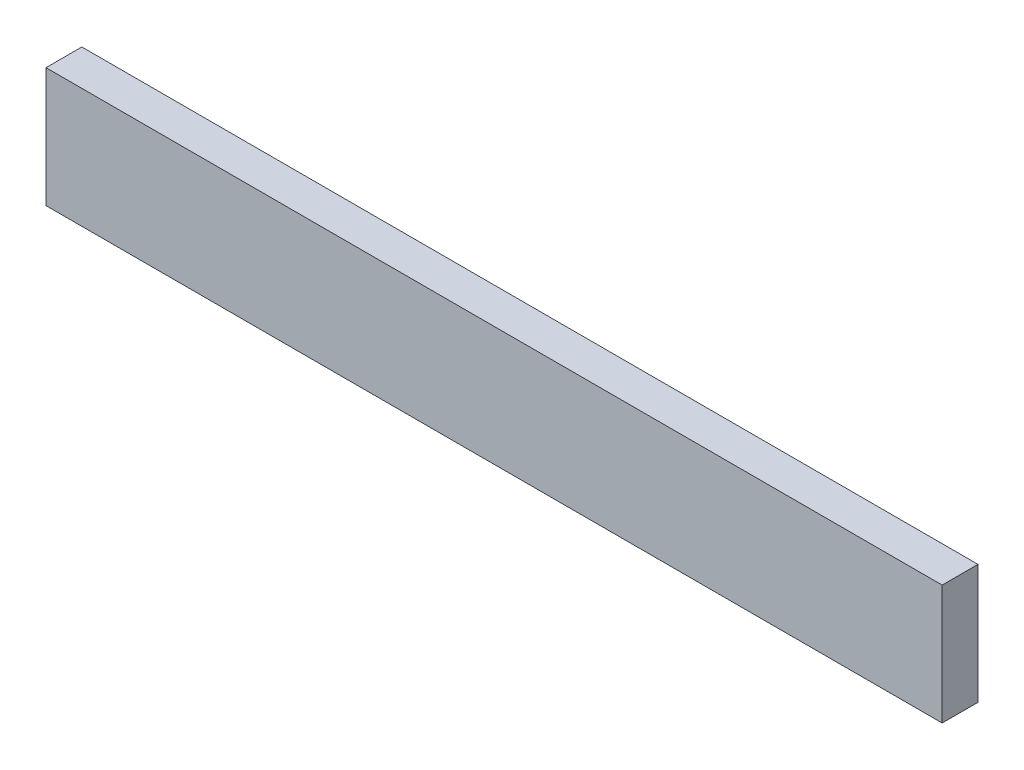
from build123d import *

# Parameters (mm, degrees)
SKETCH_1_W      = 150
SKETCH_1_H      = 20
EXTRUDE_1_DEPTH = 6


with BuildPart() as part:
    # 草图1 → 凸台-拉伸1 (new body)
    with BuildSketch(Plane.XY):
        Rectangle(SKETCH_1_W, SKETCH_1_H)
    extrude(amount=EXTRUDE_1_DEPTH)


solid = part.part
